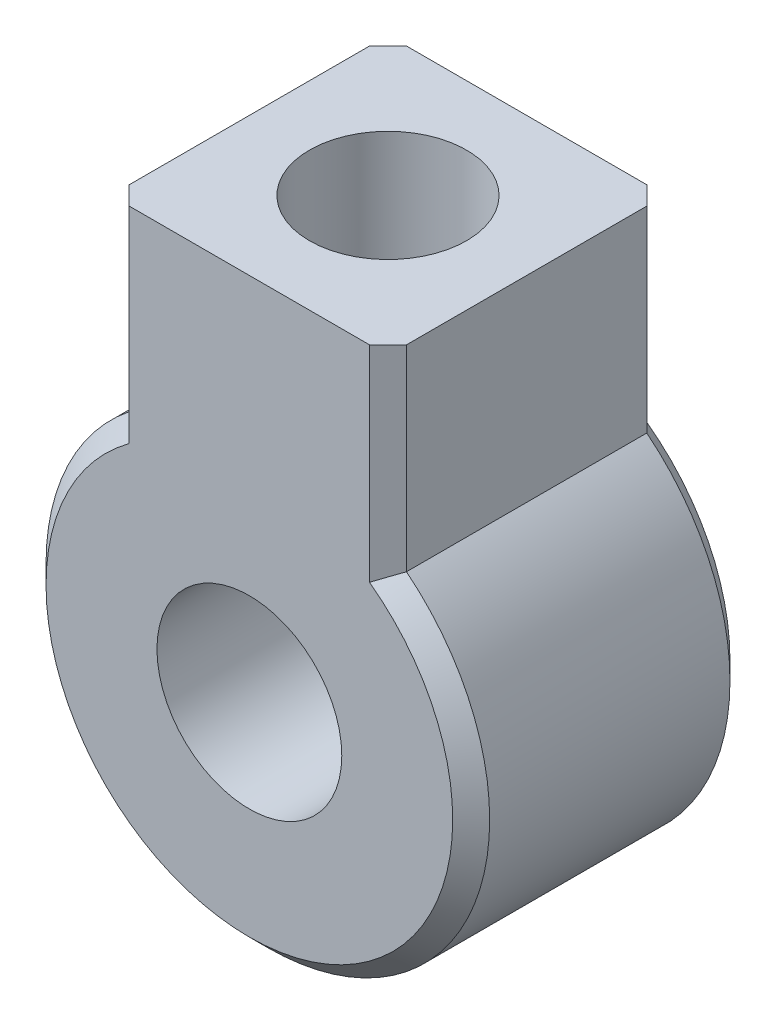
from build123d import *

# Parameters (mm, degrees)
EXTRUDE_1_DEPTH              = 15
HOLE_WIZARD_10_0_10_1_D      = 10
HOLE_WIZARD_8_5_8_5_1_REACH  = 36.989
HOLE_WIZARD_8_5_8_5_1_BORE_R = 4.25
CHAMFER_1_SIZE               = 1


with BuildPart() as part:
    # 草图1 → 凸台-拉伸1 (new body)
    with BuildSketch(Plane.XY.offset(7.5)):
        with BuildLine():
            Line((7.5, 20), (-7.5, 20))
            Line((-7.5, 20), (-7.5, 9.367496998))
            ThreePointArc((-7.5, 9.367496998), (0, -12), (7.5, 9.367496998))
            Line((7.5, 9.367496998), (7.5, 20))
        make_face()
    extrude(amount=-EXTRUDE_1_DEPTH)

    # Ø10.0 (10) 直径孔1 (through all)
    with Locations(Plane.XY.offset(7.5)):
        with Locations((0, 0)):
            Hole(HOLE_WIZARD_10_0_10_1_D / 2)

    # Ø8.5 (8.5) 直径孔1 bore → Ø8.5 (8.5) 直径孔1 (cut, up to next)
    with BuildSketch(Plane(origin=(0, 20, 0), x_dir=(1, 0, 0), z_dir=(0, 1, 0)), mode=Mode.PRIVATE) as hole_wizard_8_5_8_5_1_sk1:
        Circle(HOLE_WIZARD_8_5_8_5_1_BORE_R)
    hole_wizard_8_5_8_5_1_tool1 = extrude(hole_wizard_8_5_8_5_1_sk1.sketch, amount=-HOLE_WIZARD_8_5_8_5_1_REACH, mode=Mode.PRIVATE) & part.part
    add(hole_wizard_8_5_8_5_1_tool1.solids().sort_by_distance((0, 20, 0))[0], mode=Mode.SUBTRACT)

    # 倒角1
    chamfer_1_edges = [part.edges().sort_by_distance(p)[0] for p in [
        (-7.5, 14.683748499, -7.5),
        (0, -12, -7.5),
        (7.5, 14.683748499, -7.5),
        (0, -12, 7.5),
        (-7.5, 14.683748499, 7.5),
        (7.5, 14.683748499, 7.5),
    ]]
    chamfer(chamfer_1_edges, length=CHAMFER_1_SIZE)


solid = part.part
